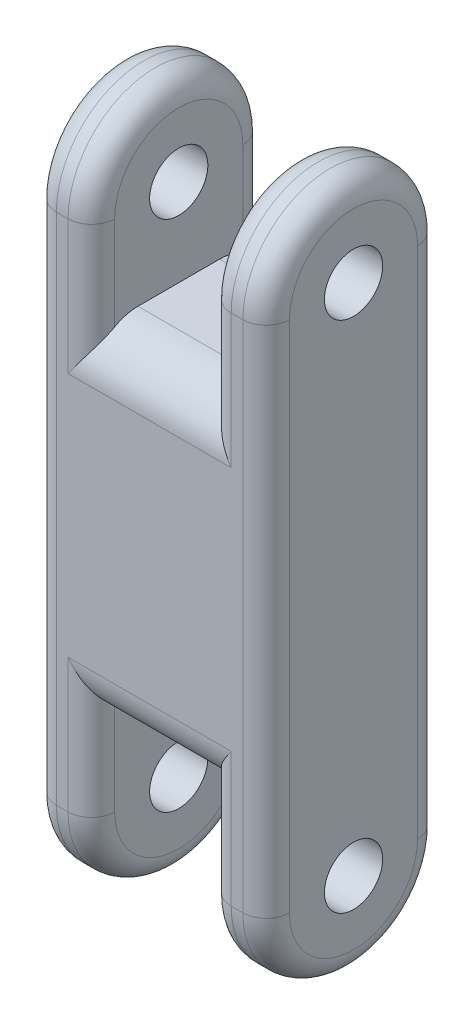
from build123d import *

# Parameters (mm, degrees)
BOSS_EXTRUDE1_DEPTH = 12.7
SKETCH2_R           = 1.5875
CUT_EXTRUDE1_DEPTH  = 19.05
CUT_EXTRUDE2_DEPTH  = 3.175
FILLET2_R           = 2.54
FILLET3_R           = 1.27
SKETCH3_R           = 1.086795662
BOSS_EXTRUDE2_DEPTH = 2.54
FILLET4_R           = 0.762
SKETCH4_R           = 0.491571792
CUT_EXTRUDE3_DEPTH  = 2.54
SCALE_RATIO_1_SCALE = 1.3


with BuildPart() as part:
    # Sketch1 → Boss-Extrude1 (new body)
    with BuildSketch(Plane(origin=(0, 0, 0), x_dir=(0, 0, -1), z_dir=(1, 0, 0))):
        with BuildLine():
            Line((-4.7625, 0), (-4.7625, 27.9908))
            ThreePointArc((-4.7625, 27.9908), (0, 32.7533), (4.7625, 27.9908))
            Line((4.7625, 27.9908), (4.7625, 0))
            ThreePointArc((4.7625, 0), (0, -4.7625), (-4.7625, 0))
        make_face()
    extrude(amount=BOSS_EXTRUDE1_DEPTH)

    # Sketch2 → Cut-Extrude1 (cut)
    with BuildSketch(Plane(origin=(12.7, 0, 0), x_dir=(0, 0, -1), z_dir=(1, 0, 0))):
        Circle(SKETCH2_R)
        with Locations((0, 27.9908)):
            Circle(SKETCH2_R)
    extrude(amount=-CUT_EXTRUDE1_DEPTH, mode=Mode.SUBTRACT)

    # 3DSketch1 → Cut-Extrude2 (cut, symmetric)
    with BuildSketch(Plane(origin=(6.35, 27.9908, -4.7625), x_dir=(0, -0.9466889316456175, 0.322149137356721), z_dir=(1, 0, 0))):
        with BuildLine():
            Line((0, 0), (4.508606037, 1.534235267))
            Line((4.508606037, 1.534235267), (7.57707657, -7.482976807))
            Line((7.57707657, -7.482976807), (3.068470533, -9.017212074))
            ThreePointArc((3.068470533, -9.017212074), (-2.97437077, -6.042841304), (0, 0))
        make_face()
        with BuildLine():
            Line((29.567051081, 0), (25.058445044, -1.534235267))
            Line((25.058445044, -1.534235267), (21.989974511, 7.482976807))
            Line((21.989974511, 7.482976807), (26.498580548, 9.017212074))
            ThreePointArc((26.498580548, 9.017212074), (32.541421852, 6.042841304), (29.567051081, 0))
        make_face()
    extrude(amount=CUT_EXTRUDE2_DEPTH, both=True, mode=Mode.SUBTRACT)

    # Fillet2
    fillet2_edges = [part.edges().sort_by_distance(p)[0] for p in [
        (6.35, 23.2283, -4.7625),
        (6.35, 4.7625, -4.7625),
        (6.35, 4.7625, 4.7625),
        (6.35, 23.2283, 4.7625),
    ]]
    fillet(fillet2_edges, radius=FILLET2_R)

    # Fillet3
    fillet3_edges = [part.edges().sort_by_distance(p)[0] for p in [
        (12.7, 32.7533, 0),
        (12.7, 13.9954, 4.7625),
        (9.525, 24.33955, 4.7625),
        (9.525, 24.33955, -4.7625),
        (3.175, 24.33955, -4.7625),
        (3.175, 24.33955, 4.7625),
        (12.7, -4.7625, 0),
        (0, 13.9954, 4.7625),
        (0, 32.7533, 0),
        (9.525, 3.65125, -4.7625),
        (9.525, 3.65125, 4.7625),
        (0, 13.9954, -4.7625),
        (3.175, 3.65125, 4.7625),
        (3.175, 3.65125, -4.7625),
        (0, -4.7625, 0),
        (12.7, 13.9954, -4.7625),
    ]]
    fillet(fillet3_edges, radius=FILLET3_R)

    # Sketch3 → Boss-Extrude2 (add)
    with BuildSketch(Plane.ZY):
        with Locations((-2.225739377, 2.096022994)):
            Circle(SKETCH3_R)
    extrude(amount=BOSS_EXTRUDE2_DEPTH)

    # Fillet4
    fillet4_edges = [part.edges().sort_by_distance(p)[0] for p in [
        (-2.54, 2.096022994, -3.312535039),
    ]]
    fillet(fillet4_edges, radius=FILLET4_R)

    # Sketch4 → Cut-Extrude3 (cut)
    with BuildSketch(Plane(origin=(0, 3.476983319, -2.007437255), x_dir=(-1, 0, 0), z_dir=(0, 0.8660254037844399, -0.4999999999999979))):
        with Locations(Location((0.856605906, -0.806785971, 0), (0, 0, 90))):
            Circle(SKETCH4_R)
    extrude(amount=-CUT_EXTRUDE3_DEPTH, mode=Mode.SUBTRACT)


with BuildPart() as part_1:
    # Scale ratio 1: scaled about (0, 0, 0)
    add(part.part.scale(SCALE_RATIO_1_SCALE))


solid = part_1.part
